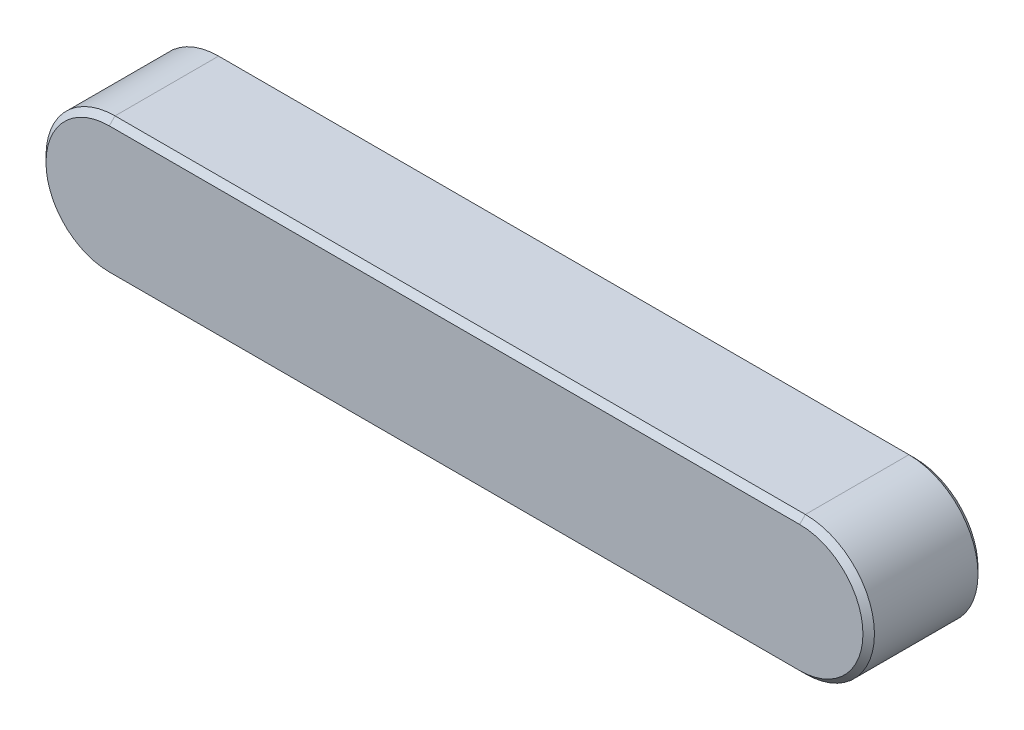
from build123d import *

# Parameters (mm, degrees)
BOSS_EXTRUDE1_DEPTH = 10
CHAMFER1_SIZE       = 0.5


with BuildPart() as part:
    # Sketch1 → Boss-Extrude1 (new body)
    with BuildSketch(Plane.XY):
        with BuildLine():
            Line((0, 6), (60, 6))
            ThreePointArc((60, 6), (66, 0), (60, -6))
            Line((60, -6), (0, -6))
            ThreePointArc((0, -6), (-6, 0), (0, 6))
        make_face()
    extrude(amount=BOSS_EXTRUDE1_DEPTH)

    # Chamfer1
    chamfer1_edges = [part.edges().sort_by_distance(p)[0] for p in [
        (66, 0, 10),
        (30, 6, 10),
        (-6, 0, 10),
        (30, 6, 0),
        (66, 0, 0),
        (30, -6, 0),
        (-6, 0, 0),
        (30, -6, 10),
    ]]
    chamfer(chamfer1_edges, length=CHAMFER1_SIZE)


solid = part.part
